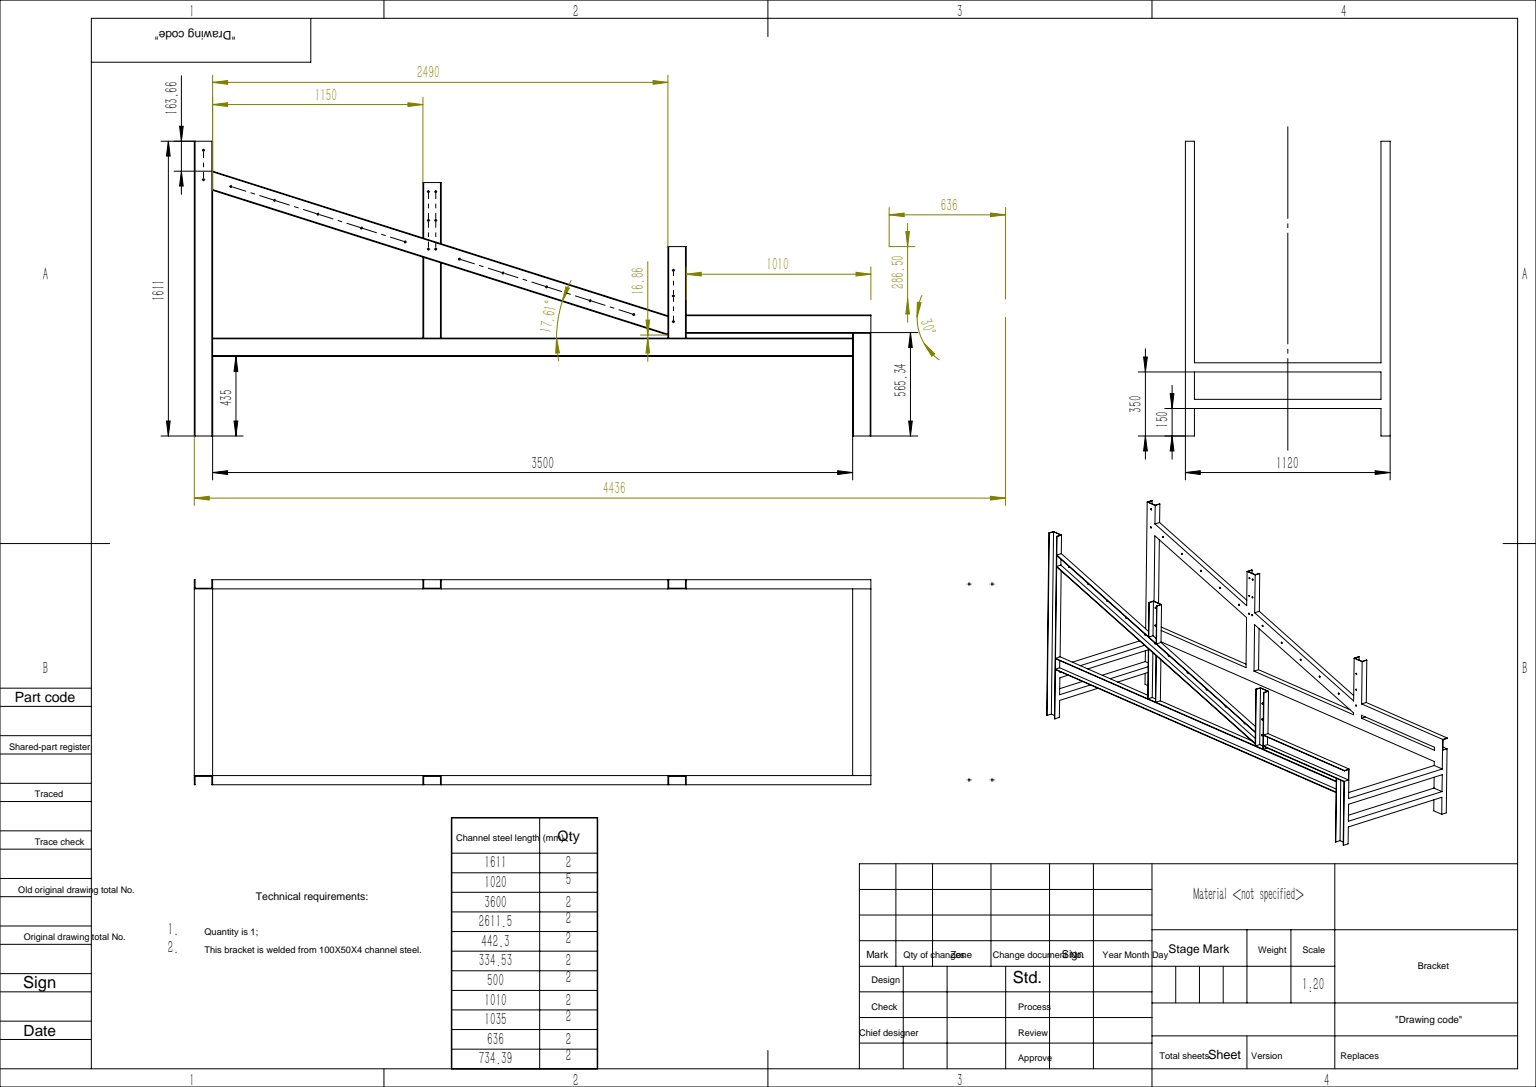
SolidWorks part; units mm, degrees
ref_plane "前视基准面" through (0, 0, 0) normal (0, 0, 1) x (1, 0, 0)
ref_plane "上视基准面" through (0, 0, 0) normal (0, 1, 0) x (1, 0, 0)
ref_plane "右视基准面" through (0, 0, 0) normal (1, 0, 0) x (0, 0, -1)
sketch "草图1" plane through (0, 0, 0) normal (0, 1, 0) x (1, 0, 0)
  line L0 (0, 0) -> (249.0872, 0) construction
  line L1 (0, -560) -> (4, -560)
  line L2 (0, -560) -> (0, -510)
  line L3 (0, -510) -> (100, -510)
  line L4 (100, -560) -> (100, -510)
  line L5 (4, -560) -> (4, -514)
  line L6 (4, -514) -> (96, -514)
  line L7 (96, -514) -> (96, -560)
  line L8 (96, -560) -> (100, -560)
  line L9 (96, 560) -> (100, 560)
  line L10 (96, 514) -> (96, 560)
  line L11 (4, 514) -> (96, 514)
  line L12 (4, 560) -> (4, 514)
  line L13 (100, 560) -> (100, 510)
  line L14 (0, 510) -> (100, 510)
  line L15 (0, 560) -> (0, 510)
  line L16 (0, 560) -> (4, 560)
extrude "凸台-拉伸1" add sketch "草图1" along normal blind 1611
sketch "草图2" plane through (100, 0, 0) normal (1, 0, 0) x (0, 0, -1)
  line L0 (-560, 1611) -> (-560, 0) construction
  line L1 (-560, 535) -> (-510, 535)
  line L2 (-560, 535) -> (-560, 531)
  line L3 (-560, 435) -> (-510, 435)
  line L4 (-510, 535) -> (-510, 435)
  line L5 (-510, 1611) -> (-510, 0) construction
  line L6 (-560, 531) -> (-514, 531)
  line L7 (-514, 531) -> (-514, 439)
  line L8 (-514, 439) -> (-560, 439)
  line L9 (-560, 439) -> (-560, 435)
  line L11 (-560, 0) -> (-510, 0) construction
  line L12 (0, 0) -> (0, 411.5694) construction
  line L13 (560, 435) -> (510, 435)
  line L14 (514, 439) -> (560, 439)
  line L15 (560, 439) -> (560, 435)
  line L16 (514, 531) -> (514, 439)
  line L17 (510, 535) -> (510, 435)
  line L18 (560, 535) -> (560, 531)
  line L19 (560, 531) -> (514, 531)
  line L20 (560, 535) -> (510, 535)
extrude "凸台-拉伸2" add sketch "草图2" along normal blind 3500
sketch "草图4" plane through (0, 535, 0) normal (0, 1, 0) x (1, 0, 0)
  line L0 (0, 0) -> (816.4724, 0) construction
  line L1 (3604, -560) -> (3604, -514)
  line L2 (3600, -560) -> (3604, -560)
  line L3 (3600, -560) -> (3600, -510)
  line L4 (3600, -510) -> (3700, -510)
  line L5 (3700, -560) -> (3700, -510)
  line L6 (3604, -514) -> (3696, -514)
  line L7 (3696, -514) -> (3696, -560)
  line L8 (3696, -560) -> (3700, -560)
  line L9 (3696, 560) -> (3700, 560)
  line L10 (3696, 514) -> (3696, 560)
  line L11 (3604, 514) -> (3696, 514)
  line L12 (3700, 560) -> (3700, 510)
  line L13 (3600, 510) -> (3700, 510)
  line L14 (3600, 560) -> (3600, 510)
  line L15 (3600, 560) -> (3604, 560)
  line L16 (3604, 560) -> (3604, 514)
extrude "凸台-拉伸3" add sketch "草图4" against normal up to vertex (535 mm away)
sketch "草图6" plane through (100, 0, 0) normal (1, 0, 0) x (0, 0, -1)
  line L0 (510, 1342.4193) -> (560, 1342.4193) construction
  line L1 (510, 1611) -> (510, 535) construction
  line L2 (560, 1611) -> (560, 535) construction
ref_plane "基准面1" through (-296.3397, 94.0865, 0) normal (0.9531, -0.3026, 0) x (0, 0, -1)
sketch "草图9" plane through (0, 535, 0) normal (0, 1, 0) x (1, 0, 0)
  line L0 (3604, 560) -> (100, 560) construction
  line L1 (2690, 560) -> (2686, 560)
  line L2 (2690, 560) -> (2690, 510)
  line L3 (2690, 510) -> (2590, 510)
  line L4 (2590, 560) -> (2590, 510)
  line L5 (3700, 510) -> (100, 510) construction
  line L6 (2686, 560) -> (2686, 514)
  line L7 (2686, 514) -> (2594, 514)
  line L8 (2594, 514) -> (2594, 560)
  line L9 (2594, 560) -> (2590, 560)
  line L11 (100, 514) -> (100, 560) construction
  point P12 (100, 537)
extrude "凸台-拉伸6" add sketch "草图9" along normal blind 500
sketch "草图10" plane through (0, 535, 0) normal (0, 1, 0) x (1, 0, 0)
  line L0 (1346, 560) -> (1346, 514)
  line L1 (1350, 560) -> (1346, 560)
  line L2 (1350, 560) -> (1350, 510)
  line L3 (1350, 510) -> (1250, 510)
  line L4 (1250, 560) -> (1250, 510)
  line L5 (1346, 514) -> (1254, 514)
  line L6 (1254, 514) -> (1254, 560)
  line L7 (1254, 560) -> (1250, 560)
  line L8 (2590, 560) -> (100, 560) construction
  line L9 (2590, 510) -> (100, 510) construction
  line L10 (100, 560) -> (100, 510) construction
extrude "凸台-拉伸7" add sketch "草图10" along normal blind 850
sketch "草图8" plane through (-296.3397, 94.0865, 0) normal (0.9531, -0.3026, 0) x (0, 0, -1)
  line L0 (560, 1405.7404) -> (514, 1405.7404)
  line L1 (560, 1309.7404) -> (510, 1309.7404)
  line L2 (560, 1309.7404) -> (560, 1313.7404)
  line L3 (560, 1409.7404) -> (510, 1409.7404)
  line L4 (510, 1309.7404) -> (510, 1409.7404)
  line L5 (514, 1405.7404) -> (514, 1313.7404)
  line L6 (514, 1313.7404) -> (560, 1313.7404)
  line L7 (560, 1405.7404) -> (560, 1409.7404)
extrude "凸台-拉伸5" add sketch "草图8" along normal up to surface and the other way up to surface up to face at (2590, 785, -535) other way up to face at (100, 1342, -541.25)
sketch "草图12" plane through (0, 0, -510) normal (0, 0, 1) x (1, 0, 0)
  line L0 (3600, 0) -> (3700, 0) construction
  line L1 (3600, 400) -> (3700, 400)
  line L2 (3600, 400) -> (3600, 350)
  line L3 (3600, 350) -> (3604, 350)
  line L4 (3700, 400) -> (3700, 350)
  line L5 (3700, 0) -> (3700, 535) construction
  line L6 (3604, 350) -> (3604, 396)
  line L7 (3604, 396) -> (3696, 396)
  line L8 (3696, 396) -> (3696, 350)
  line L9 (3696, 350) -> (3700, 350)
  line L12 (3600, 439) -> (3600, 531) construction
extrude "凸台-拉伸8" add sketch "草图12" along normal up to surface (1020 mm away) up to face at (1855, 570, 510)
sketch "草图22" plane through (-296.3397, 94.0865, 0) normal (0.9531, -0.3026, 0) x (0, 0, -1)
  line L0 (560, 1405.7404) -> (560, 1313.7404) construction
  line L1 (560, 1313.7404) -> (514, 1313.7404)
  line L2 (560, 1313.7404) -> (560, 1405.7404)
  line L3 (560, 1405.7404) -> (514, 1405.7404)
  line L4 (514, 1313.7404) -> (514, 1405.7404)
  line L5 (514, 1313.7404) -> (514, 1405.7404) construction
  line L6 (514, 1405.7404) -> (560, 1405.7404) construction
  line L7 (560, 1313.7404) -> (514, 1313.7404) construction
extrude "切除-拉伸5" cut sketch "草图22" along normal blind 1500
sketch "草图30" plane through (2690, 0, 0) normal (1, 0, 0) x (0, 0, -1)
  line L0 (560, 657.3394) -> (514, 657.3394)
  line L1 (510, 661.3394) -> (560, 661.3394)
  line L2 (510, 661.3394) -> (510, 561.3394)
  line L3 (510, 561.3394) -> (560, 561.3394)
  line L4 (560, 661.3394) -> (560, 657.3394)
  line L5 (514, 657.3394) -> (514, 565.3394)
  line L6 (514, 565.3394) -> (560, 565.3394)
  line L7 (560, 565.3394) -> (560, 561.3394)
  line L8 (510, 661.3394) -> (558, 661.3394) construction
  line L9 (510, 1035) -> (510, 535) construction
extrude "凸台-拉伸9" add sketch "草图30" along normal up to surface (1010 mm away) contours L1 L4 L0 L5 L6 L7 L3 L2 up to face at (3700, 262.9167, 85)
sketch "草图5" plane through (0, 535, 0) normal (0, 1, 0) x (1, 0, 0)
  line L1 (3600, 560) -> (3600, 510) construction
  line L2 (3604, 560) -> (3600, 560) construction
  line L3 (3696, 514) -> (3604, 514) construction
  line L4 (3600, 510) -> (3700, 510) construction
  line L5 (3700, 510) -> (3700, 560) construction
  line L6 (3700, 560) -> (3696, 560) construction
  line L7 (3696, 560) -> (3696, 514) construction
  line L8 (3600, 560) -> (3600, 510)
  line L9 (3604, 560) -> (3600, 560)
  line L10 (3696, 514) -> (3604, 514)
  line L11 (3600, 510) -> (3700, 510)
  line L12 (3700, 510) -> (3700, 560)
  line L13 (3700, 560) -> (3696, 560)
  line L14 (3696, 560) -> (3696, 514)
  line L22 (3604, 514) -> (3604, 560) construction
  line L23 (3604, 514) -> (3604, 560)
extrude "凸台-拉伸4" add sketch "草图5" along normal up to surface (26.3394 mm away) up to face at (3195, 561.3394, -535)
sketch "草图20" plane through (0, 0, -514) normal (0, 0, -1) x (-1, 0, 0)
  line L0 (0, 1611) -> (0, 0) construction
  line L2 (-96, 1611) -> (-4, 1611) construction
  circle A0 centre (-50, 1561) radius 5
  dimension "D1" = 10
  dimension "D2" = 50
  dimension "D3" = 50
extrude "切除-拉伸3" cut sketch "草图20" against normal through all
pattern_linear "阵列(线性)1" count 2 spacing 160 along (0, -1, 0) of "切除-拉伸3"
sketch "草图21" plane through (0, 0, -514) normal (0, 0, -1) x (-1, 0, 0)
  line L0 (-1250, 977.2997) -> (-100, 1342.4193) construction
  line L3 (-100, 1342.4193) -> (-100, 535) construction
  circle A0 centre (-200, 1363.1293) radius 5
  dimension "D3" = 10
  dimension "D1" = 50
  dimension "D2" = 100
extrude "切除-拉伸4" cut sketch "草图21" against normal through all
pattern_linear "阵列(线性)2" count 5 spacing 250 along (0.9531, -0.3026, 0) of "切除-拉伸4"
sketch "草图23" plane through (0, 0, -514) normal (0, 0, -1) x (-1, 0, 0)
  line L0 (-1250, 1385) -> (-1250, 1082.2189) construction
  line L1 (-1350, 1385) -> (-1350, 1050.4694) construction
  line L2 (-1346, 1385) -> (-1254, 1385) construction
  circle A0 centre (-1280, 1335) radius 5
  circle A1 centre (-1320, 1335) radius 5
  dimension "D1" = 10
  dimension "D2" = 30
  dimension "D3" = 30
  dimension "D4" = 50
extrude "切除-拉伸6" cut sketch "草图23" against normal through all
pattern_linear "阵列(线性)3" count 3 spacing 157 along (0, -1, 0) of "切除-拉伸6"
sketch "草图24" plane through (0, 0, -514) normal (0, 0, -1) x (-1, 0, 0)
  line L0 (-1350, 945.5502) -> (-1350, 535) construction
  line L1 (-2590, 551.8561) -> (-1350, 945.5502) construction
  circle A0 centre (-1450, 966.2603) radius 5
  dimension "D1" = 10
  dimension "D2" = 100
  dimension "D3" = 50
extrude "切除-拉伸7" cut sketch "草图24" against normal through all
pattern_linear "阵列(线性)4" count 5 spacing 250 along (0.9531, -0.3026, 0) of "切除-拉伸7"
sketch "草图25" plane through (0, 0, -514) normal (0, 0, -1) x (-1, 0, 0)
  line L1 (-2590, 1035) -> (-2590, 656.7752) construction
  line L3 (-2594, 1035) -> (-2590, 1035) construction
  circle A0 centre (-2620, 905) radius 5
  dimension "D4" = 10
  dimension "D1" = 130
  dimension "D2" = 30
extrude "切除-拉伸8" cut sketch "草图25" against normal through all
pattern_linear "阵列(线性)5" count 3 spacing 140 along (0, -1, 0) of "切除-拉伸8"
pattern_linear "阵列(线性)8" count 2 spacing 200 along (0, -1, 0) count 2 spacing 3600 along (-1, 0, 0) of "凸台-拉伸8"
mirror "镜向7" about plane through (0, 0, 0) normal (0, 0, 1) of "阵列(线性)5", "凸台-拉伸4", "凸台-拉伸6", "凸台-拉伸7", "凸台-拉伸5", "切除-拉伸5", "凸台-拉伸9", "阵列(线性)1", "切除-拉伸3", "切除-拉伸4", "阵列(线性)2", "切除-拉伸6", "阵列(线性)3", "切除-拉伸7", "阵列(线性)4", "切除-拉伸8"
equation "\"a1\"= 100'槽钢H"
equation "\"a2\"= 50'槽钢B"
equation "\"a3\"= 4'槽钢t"
equation "\"a4\"= 1020'支架内侧的距离"
equation "\"a5\"= 3500'支架长度方向的槽钢长度"
equation "\"D1@草图1\"=\"a1\""
equation "\"D2@草图1\"=\"a2\""
equation "\"D3@草图1\"=\"a3\""
equation "\"D4@草图1\"=\"a3\""
equation "\"D5@草图1\"=\"a4\"/2"
equation "\"D2@草图2\"=\"a1\""
equation "\"D3@草图2\"=\"a3\""
equation "\"D4@草图2\"=\"a3\""
equation "\"D1@凸台-拉伸2\"=\"a5\""
equation "\"D1@草图4\"=\"a2\""
equation "\"D2@草图4\"=\"a3\""
equation "\"D3@草图4\"=\"a1\""
equation "\"D4@草图4\"=\"a3\""
equation "\"D1@草图8\"=\"a1\""
equation "\"D2@草图8\"=\"a3\""
equation "\"D3@草图8\"=\"a3\""
equation "\"D4@草图8\"=\"a2\""
equation "\"D2@草图9\"=\"a3\""
equation "\"D3@草图9\"=\"a3\""
equation "\"D4@草图9\"=\"a1\""
equation "\"D1@草图10\"=\"a1\""
equation "\"D2@草图10\"=\"a3\""
equation "\"D3@草图10\"=\"a3\""
equation "\"D1@草图12\"=\"a2\""
equation "\"D2@草图12\"=\"a3\""
equation "\"D3@草图12\"=\"a3\""
equation "\"D1@草图30\"=\"a3\""
equation "\"D2@草图30\"=\"a3\""
equation "\"D3@草图30\"=\"a1\""
equation "\"D4@草图30\"=\"a2\""
equation "\"D4@阵列(线性)8\"=\"a5\"+\"a1\""
